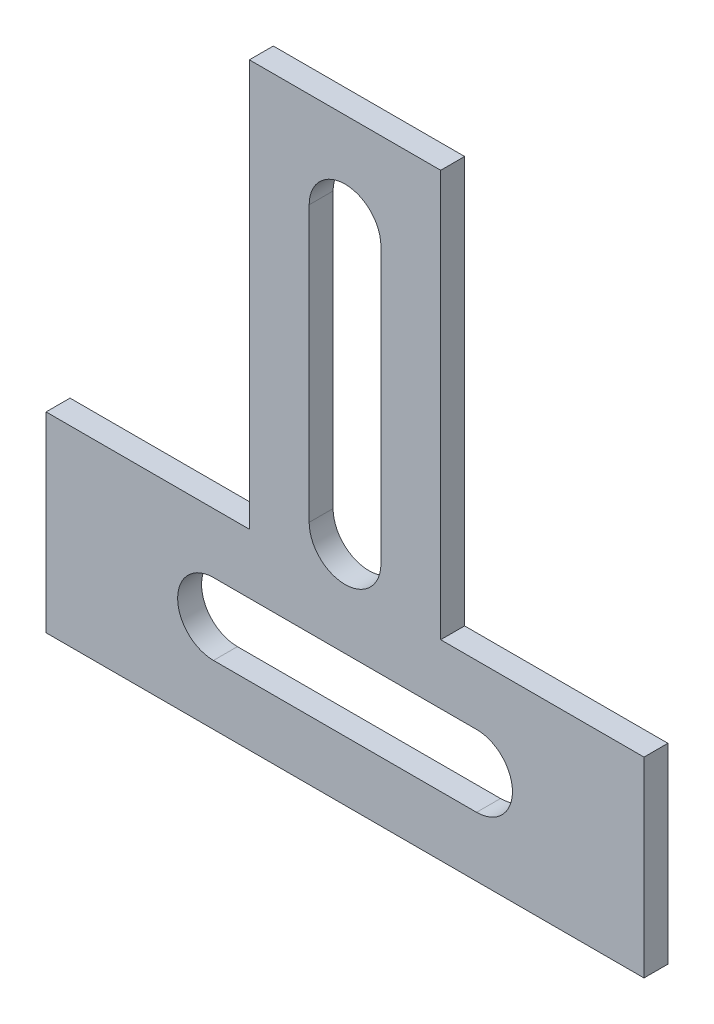
from build123d import *

# Parameters (mm, degrees)
EXTRUDE_2_DEPTH = 2


with BuildPart() as part:
    # 草图1 → 凸台-拉伸2 (new body)
    with BuildSketch(Plane.XY):
        Polygon((25, -8), (-25, -8), (-25, 8), (-8, 8), (-8, 42), (8, 42), (8, 8), (25, 8), align=None)
        with BuildLine():
            Line((-3, 11), (-3, 34))
            ThreePointArc((-3, 34), (0, 37), (3, 34))
            Line((3, 34), (3, 11))
            ThreePointArc((3, 11), (0, 8), (-3, 11))
        make_face(mode=Mode.SUBTRACT)
        with BuildLine():
            Line((-11, 3), (11, 3))
            ThreePointArc((11, 3), (14, 0), (11, -3))
            Line((11, -3), (-11, -3))
            ThreePointArc((-11, -3), (-14, 0), (-11, 3))
        make_face(mode=Mode.SUBTRACT)
    extrude(amount=EXTRUDE_2_DEPTH)


solid = part.part
